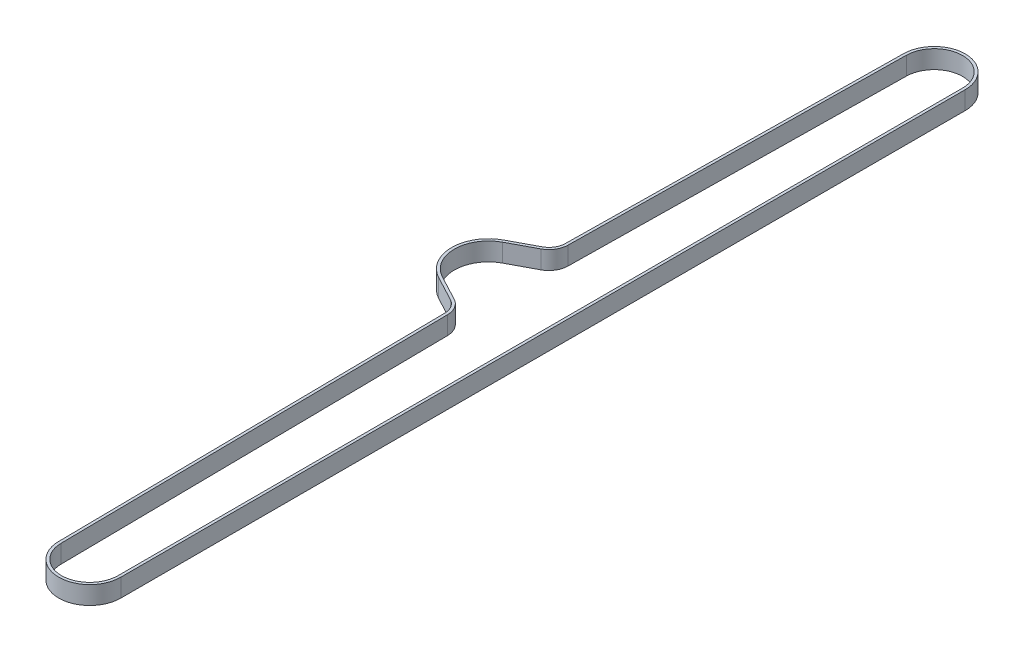
SolidWorks part; units mm, degrees
ref_plane "前视基准面" through (0, 0, 0) normal (0, 0, 1) x (1, 0, 0)
ref_plane "上视基准面" through (0, 0, 0) normal (0, 1, 0) x (1, 0, 0)
ref_plane "右视基准面" through (0, 0, 0) normal (1, 0, 0) x (0, 0, -1)
sketch "草图1" plane through (-54.3898, 234.4596, 1948) normal (0, -1, 0) x (0, 0, 1)
  line L0 (-1396, -47.745) -> (0, -47.745)
  line L1 (-1396.6719, 47.7403) -> (-845.0638, 55.5031)
  line L2 (-818.1285, 71.9465) -> (-796.0886, 113.3981)
  line L3 (-694.9114, 113.3981) -> (-672.8714, 71.9465)
  line L4 (0.5731, 47.7416) -> (-645.8721, 55.5022)
  arc A0 (0, -47.745) -> (0.5731, 47.7416) centre (0, 0) ccw
  arc A1 (-1396.6719, 47.7403) -> (-1396, -47.745) centre (-1396, 0) ccw
  arc A2 (-694.9114, 113.3981) -> (-796.0886, 113.3981) centre (-745.5, 86.5) ccw
  arc A3 (-845.0638, 55.5031) -> (-818.1285, 71.9465) centre (-845.5, 86.5) ccw
  arc A4 (-672.8714, 71.9465) -> (-645.8721, 55.5022) centre (-645.5, 86.5) ccw
  dimension "D1" = 95.49
  dimension "D2" = 95.49
  dimension "D3" = 114.59
  dimension "D4" = 62
  dimension "D5" = 62
extrude "拉伸-薄壁1" add sketch "草图1" along normal mid plane 30 thin contours L0 A1 L1 A3 L2 A2 L3 A4 L4
